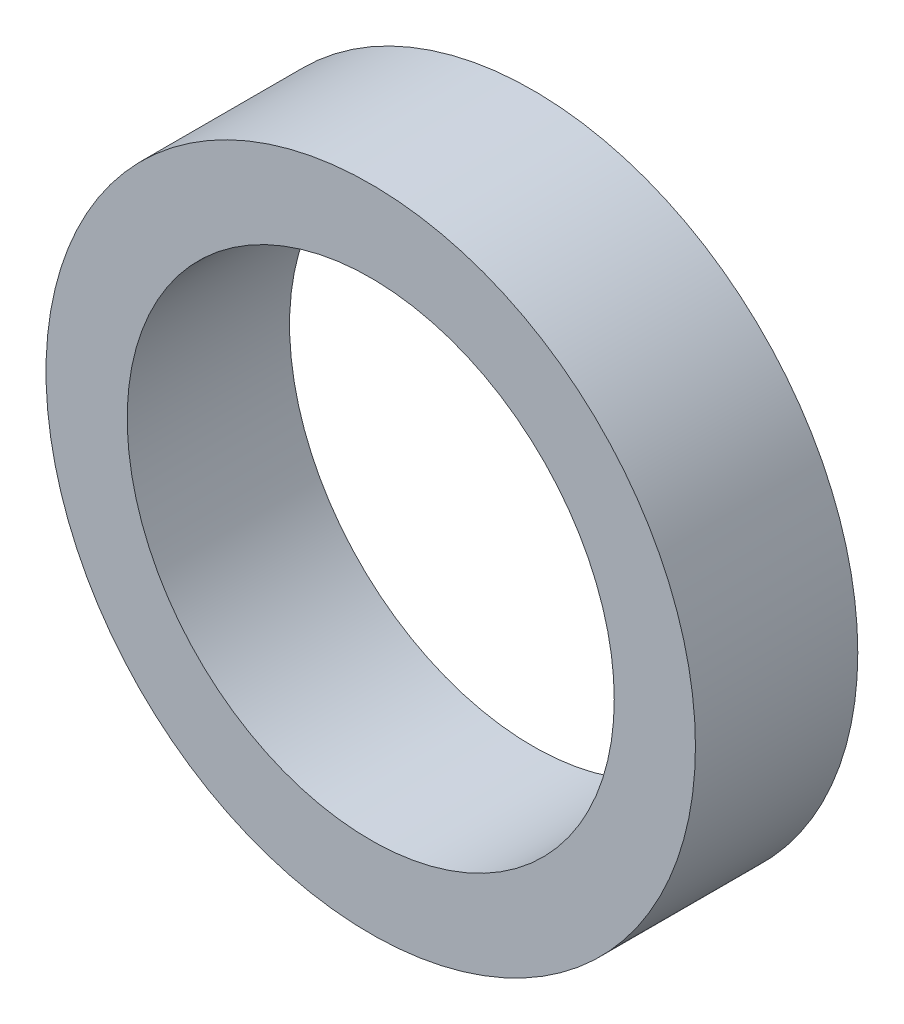
from build123d import *

# Parameters (mm, degrees)
SKETCH1_R           = 4
SKETCH1_R_2         = 3
BOSS_EXTRUDE1_DEPTH = 2


with BuildPart() as part:
    # Sketch1 → Boss-Extrude1 (new body)
    with BuildSketch(Plane.XY):
        Circle(SKETCH1_R)
        Circle(SKETCH1_R_2, mode=Mode.SUBTRACT)
    extrude(amount=BOSS_EXTRUDE1_DEPTH)


solid = part.part
